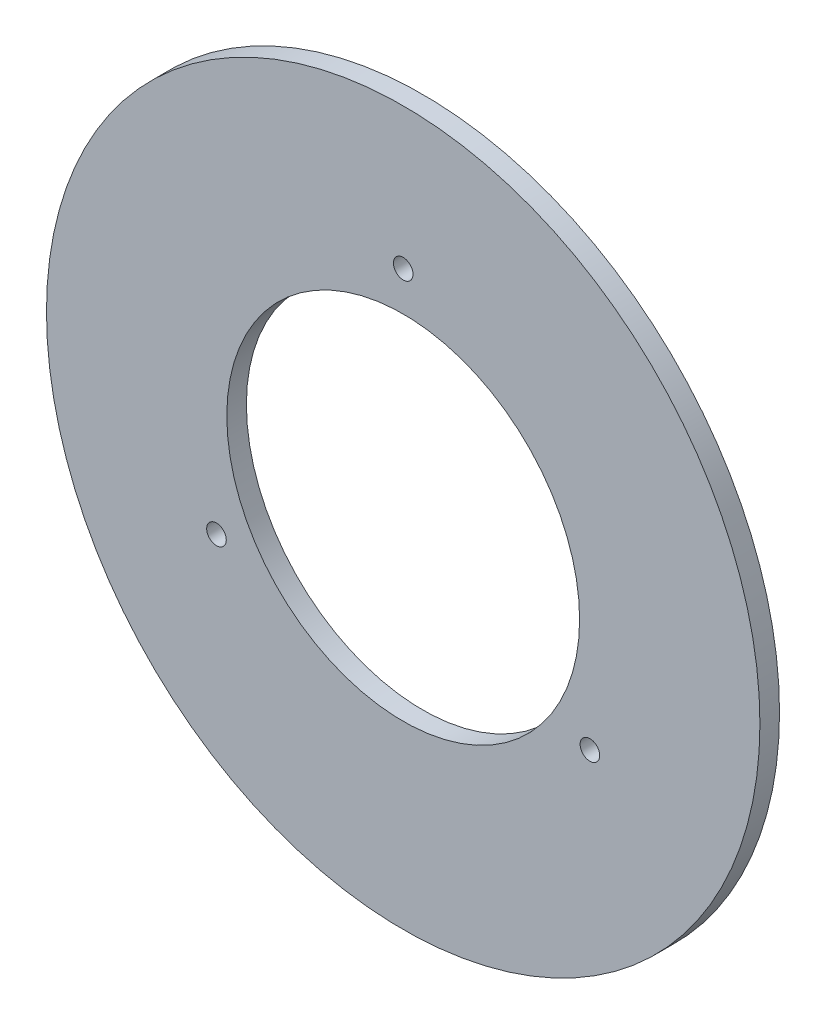
from build123d import *

# Parameters (mm, degrees)
SKETCH1_R           = 91
SKETCH1_R_2         = 45
SKETCH1_R_3         = 2.5
BOSS_EXTRUDE1_DEPTH = 5


with BuildPart() as part:
    # Sketch1 → Boss-Extrude1 (new body)
    with BuildSketch(Plane.XY):
        Circle(SKETCH1_R)
        Circle(SKETCH1_R_2, mode=Mode.SUBTRACT)
        with Locations((0, 55)):
            Circle(SKETCH1_R_3, mode=Mode.SUBTRACT)
        with Locations((47.631397208, -27.5)):
            Circle(SKETCH1_R_3, mode=Mode.SUBTRACT)
        with Locations((-47.631397208, -27.5)):
            Circle(SKETCH1_R_3, mode=Mode.SUBTRACT)
    extrude(amount=BOSS_EXTRUDE1_DEPTH)


solid = part.part
